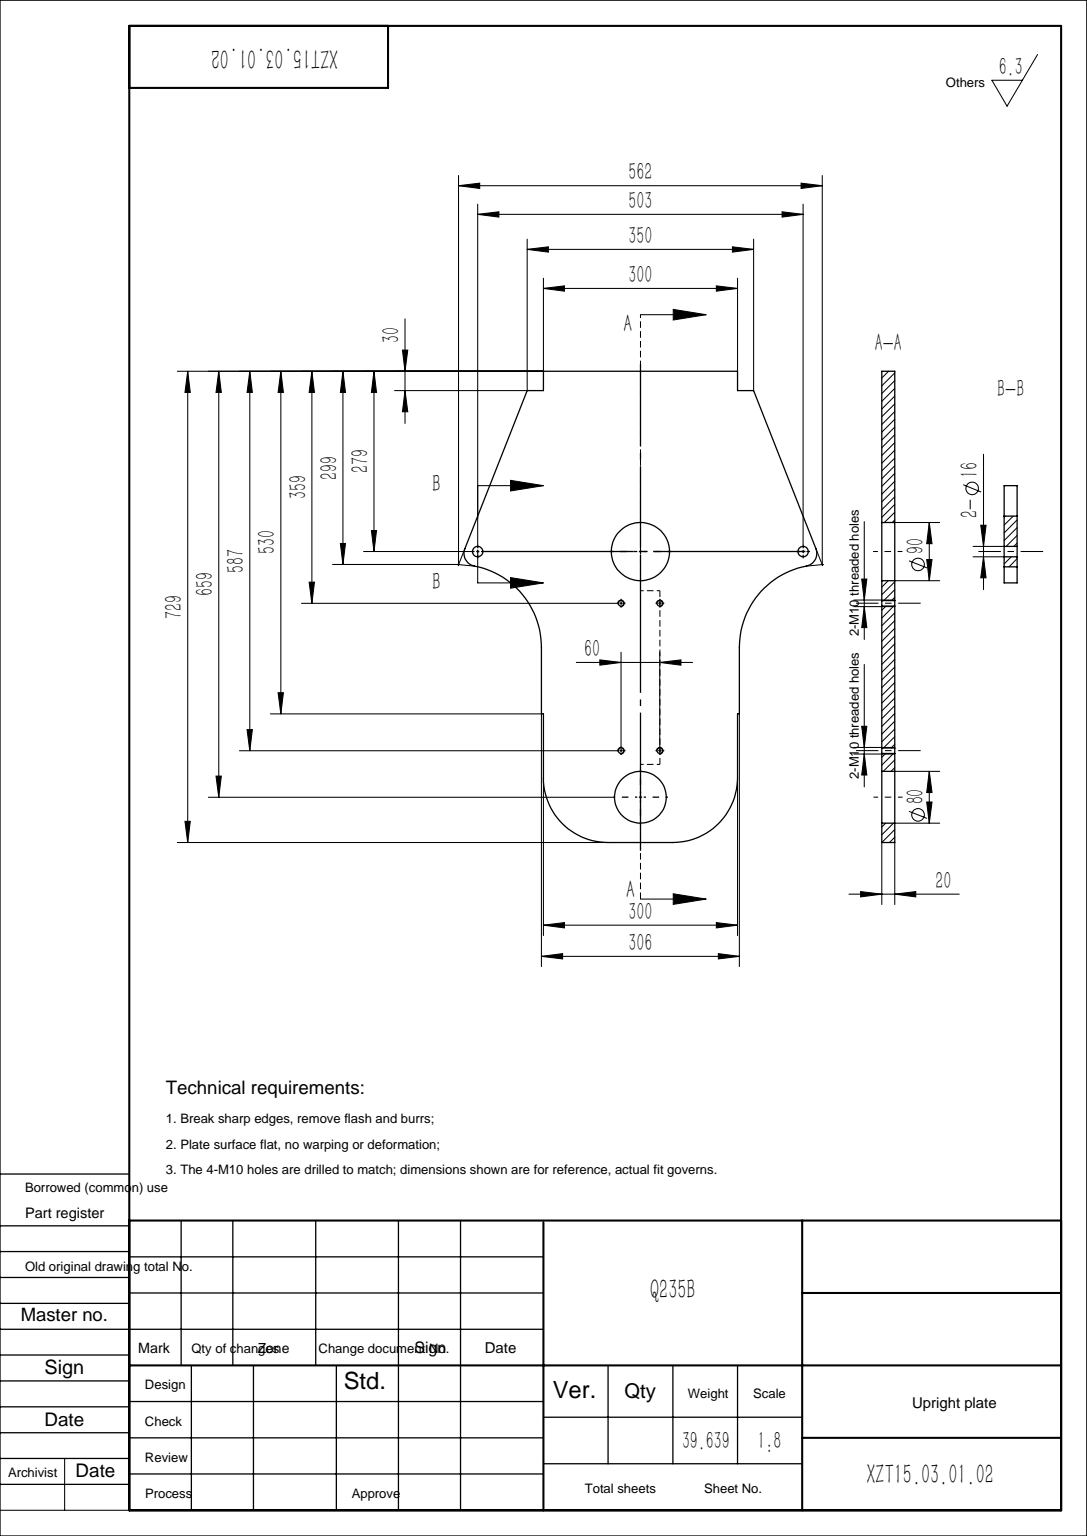
from build123d import *

# Parameters (mm, degrees)
SKETCH1_R           = 45
SKETCH1_R_2         = 40
SKETCH1_R_3         = 8
BOSS_EXTRUDE1_DEPTH = 20
FILLET1_R           = 100
FILLET2_R           = 20
M10_TAPPED_HOLE1_D  = 8.5


with BuildPart() as part:
    # Sketch1 → Boss-Extrude1 (new body)
    with BuildSketch(Plane.XY):
        with BuildLine():
            Line((-150, 0), (150, 0))
            Line((150, 0), (150, 199))
            Line((150, 199), (153, 199))
            Line((153, 199), (153, 302))
            ThreePointArc((153, 302), (190.490332008, 392.509667992), (281, 430))
            Line((281, 430), (175, 699))
            Line((175, 699), (150, 699))
            Line((150, 699), (150, 729))
            Line((150, 729), (-150, 729))
            Line((-150, 729), (-150, 699))
            Line((-150, 699), (-175, 699))
            Line((-175, 699), (-281, 430))
            ThreePointArc((-281, 430), (-190.490332008, 392.509667992), (-153, 302))
            Line((-153, 302), (-153, 199))
            Line((-153, 199), (-150, 199))
            Line((-150, 199), (-150, 0))
        make_face()
        with Locations((0, 450)):
            Circle(SKETCH1_R, mode=Mode.SUBTRACT)
        with Locations((0, 70)):
            Circle(SKETCH1_R_2, mode=Mode.SUBTRACT)
        with Locations((-251.5, 450)):
            Circle(SKETCH1_R_3, mode=Mode.SUBTRACT)
        with Locations(Location((251.5, 450, 0), (0, 0, 180))):
            Circle(SKETCH1_R_3, mode=Mode.SUBTRACT)
    extrude(amount=BOSS_EXTRUDE1_DEPTH)

    # Fillet1
    fillet1_edges = [part.edges().sort_by_distance(p)[0] for p in [
        (150, 0, 10),
        (-150, 0, 10),
    ]]
    fillet(fillet1_edges, radius=FILLET1_R)

    # Fillet2
    fillet2_edges = [part.edges().sort_by_distance(p)[0] for p in [
        (-281, 430, 10),
        (281, 430, 10),
    ]]
    fillet(fillet2_edges, radius=FILLET2_R)

    # M10 Tapped Hole1 (through all)
    with Locations(Plane.XY.offset(20)):
        with Locations((-30, 370), (-30, 142), (30, 142), (30, 370)):
            Hole(M10_TAPPED_HOLE1_D / 2)


solid = part.part
